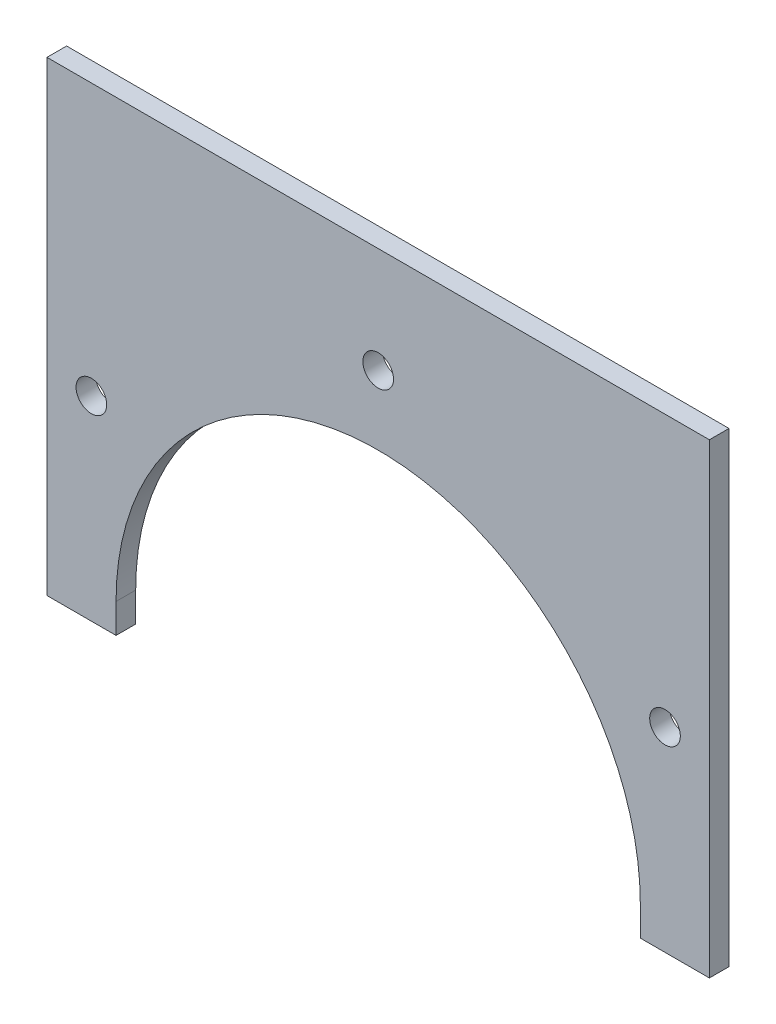
from build123d import *

# Parameters (mm, degrees)
BOSS_EXTRUDE1_DEPTH = 8
SKETCH2_R           = 6.25
CUT_EXTRUDE1_DEPTH  = 224.546415762


with BuildPart() as part:
    # Sketch1 → Boss-Extrude1 (new body)
    with BuildSketch(Plane(origin=(0, 0, 0), x_dir=(-1, 0, 0), z_dir=(0, 0, 1))):
        with BuildLine():
            Line((-106.85, 12), (-135, 12))
            Line((-135, 12), (-135, -178))
            Line((-135, -178), (135, -178))
            Line((135, -178), (135, 12))
            Line((135, 12), (106.85, 12))
            Line((106.85, 12), (106.85, 0))
            ThreePointArc((106.85, 0), (0, -106.85), (-106.85, 0))
            Line((-106.85, 0), (-106.85, 12))
        make_face()
    extrude(amount=BOSS_EXTRUDE1_DEPTH)

    # Sketch2 → Cut-Extrude1 (cut, through all)
    with BuildSketch(Plane(origin=(0, 0, 0), x_dir=(-1, 0, 0), z_dir=(0, 0, -1))):
        with Locations((-116.913429511, 67.5)):
            Circle(SKETCH2_R)
        with Locations((116.913429511, 67.5)):
            Circle(SKETCH2_R)
        with Locations((0, 135)):
            Circle(SKETCH2_R)
    extrude(amount=-CUT_EXTRUDE1_DEPTH, mode=Mode.SUBTRACT)


solid = part.part
